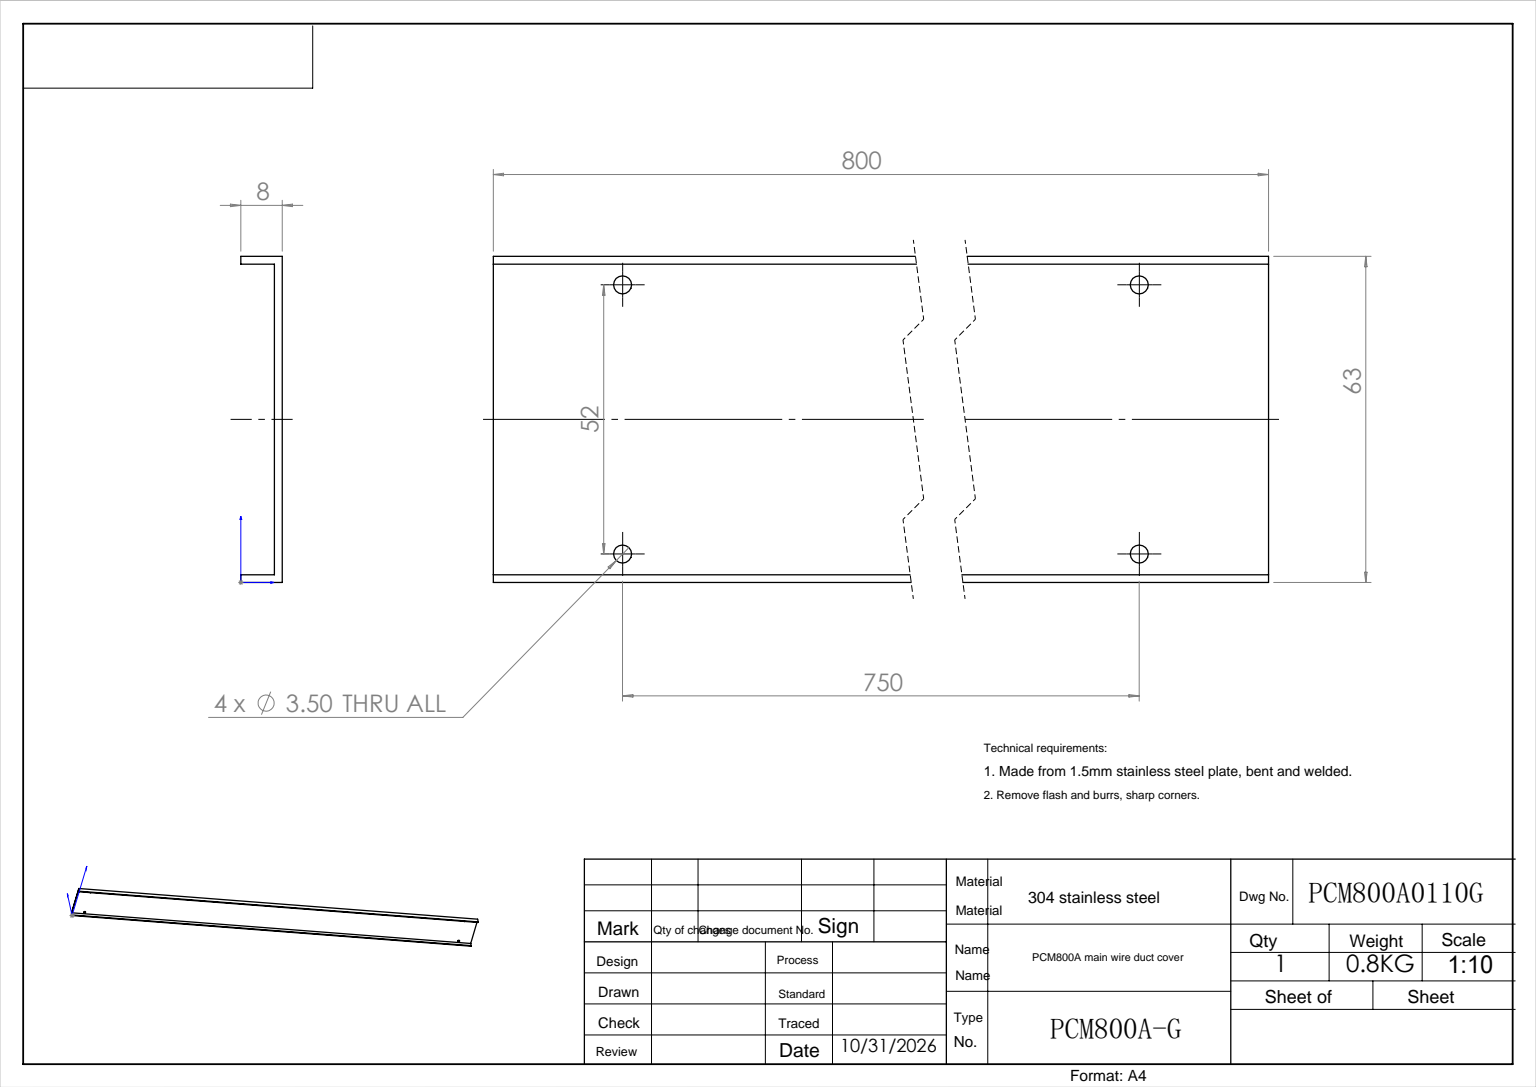
SolidWorks part; units mm, degrees
ref_plane "前视基准面" through (0, 0, 0) normal (0, 0, 1) x (1, 0, 0)
ref_plane "上视基准面" through (0, 0, 0) normal (0, 1, 0) x (1, 0, 0)
ref_plane "右视基准面" through (0, 0, 0) normal (1, 0, 0) x (0, 0, -1)
sketch "草图1" plane through (0, 0, 0) normal (0, 0, 1) x (1, 0, 0)
  line L0 (0, 0) -> (8, 0)
  line L1 (8, 0) -> (8, 63)
  line L2 (8, 63) -> (0, 63)
  dimension "D1" = 63
  dimension "D2" = 8
  dimension "D3" = 8
extrude "拉伸-薄壁1" add sketch "草图1" along normal blind 800 thin thin type one direction reverse wall 1.5
hole_wizard "Ø3.5 (3.5) 直径孔1" positions "草图3" profile "草图2" hole size "Ø3.5" standard "GB" end condition through all
sketch "草图3" plane through (8, 0, 0) normal (1, 0, 0) x (0, 0, -1)
  line L0 (-800, 0) -> (-800, 63) construction
  line L1 (-800, 63) -> (0, 63) construction
  line L2 (0, 1.5) -> (0, 61.5) construction
  point P0 (-775, 57.5)
  point P1 (-25, 57.5)
  dimension "D1" = 25
  dimension "D2" = 25
  dimension "D3" = 5.5
  dimension "D4" = 5.5
sketch "草图2" plane through (8, 57.5, 775) normal (0, 1, 0) x (0, 0, -1)
  line L0 (0, 0) -> (0, 8)
  line L1 (0, 8) -> (1.75, 8)
  line L2 (1.75, 8) -> (1.75, 0)
  line L5 (1.75, 0) -> (0, 0)
  line L11 (0, -6.35) -> (0, 107.95) construction
  dimension "通孔孔直径" = 3.5
  dimension "通孔孔深度" = 8
ref_plane "基准面1" through (0, 31.5, 0) normal (0, -1, 0) x (1, 0, 0)
mirror "镜向1" about plane through (0, 31.5, 0) normal (0, -1, 0) of "Ø3.5 (3.5) 直径孔1"
